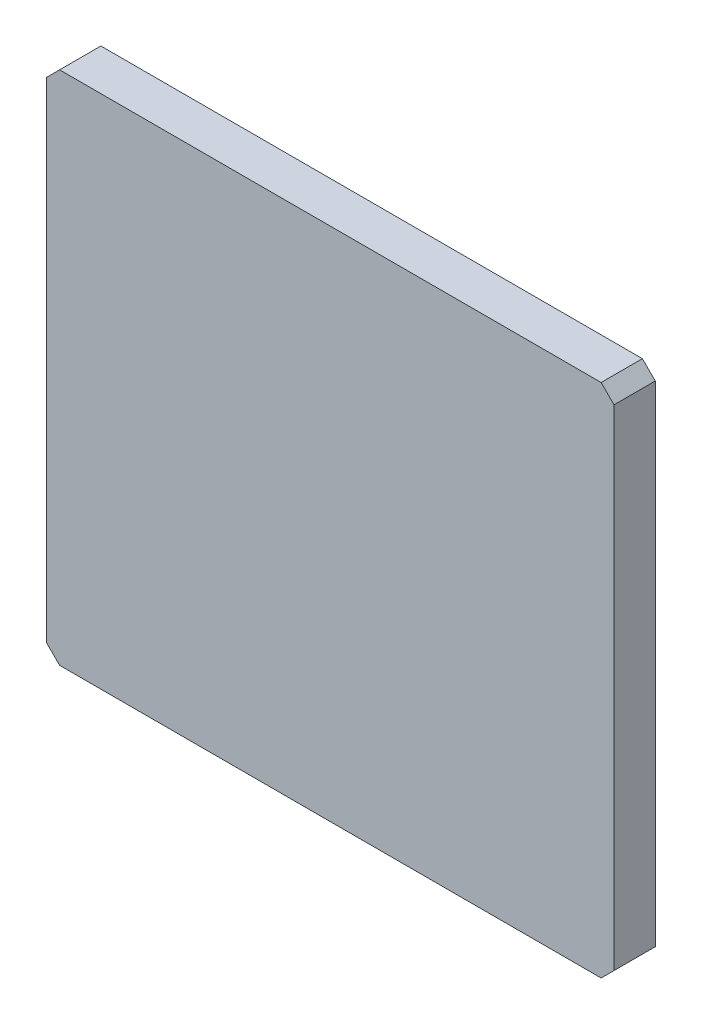
from build123d import *

# Parameters (mm, degrees)
SKETCH_1_W      = 220
SKETCH_1_H      = 200
EXTRUDE_1_DEPTH = 16
CHAMFER_1_SIZE  = 5


with BuildPart() as part:
    # 草图1 → 凸台-拉伸1 (new body)
    with BuildSketch(Plane.XY):
        with Locations((110, -100)):
            Rectangle(SKETCH_1_W, SKETCH_1_H)
    extrude(amount=EXTRUDE_1_DEPTH)

    # 倒角1
    chamfer_1_edges = [part.edges().sort_by_distance(p)[0] for p in [
        (0, 0, 8),
        (220, 0, 8),
        (220, -200, 8),
        (0, -200, 8),
    ]]
    chamfer(chamfer_1_edges, length=CHAMFER_1_SIZE)


solid = part.part
